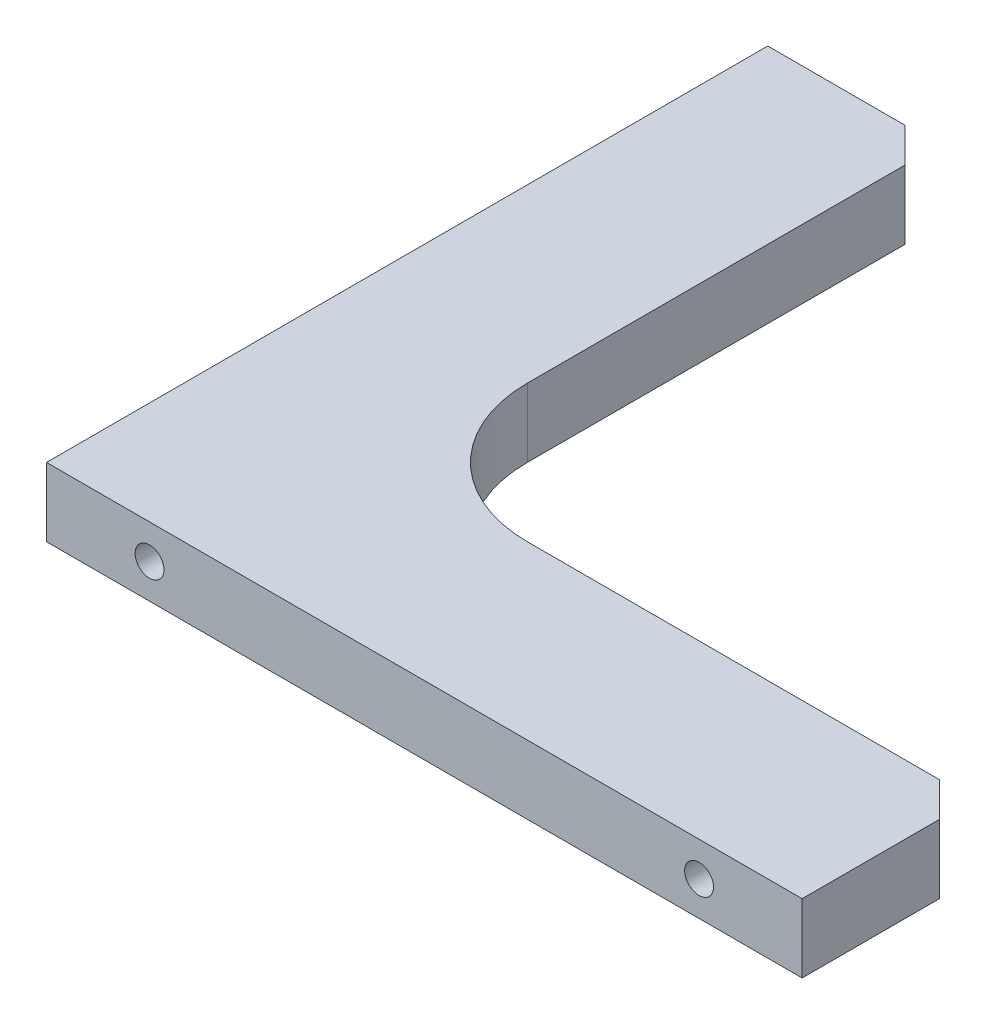
from build123d import *

# Parameters (mm, degrees)
SKETCH_1_W                  = 110
SKETCH_1_H                  = 105
EXTRUDE_1_DEPTH             = 5
CUT_EXTRUDE_1_DEPTH         = 10
CHAMFER_1_SIZE              = 5
HOLE_WIZARD_M5_1_AT_2_COUNT = 2
HOLE_WIZARD_M5_1_AT_2_PITCH = 80


with BuildPart() as part:
    # 草图1 → 凸台-拉伸1 (new, symmetric)
    with BuildSketch(Plane(origin=(0, 0, 0), x_dir=(1, 0, 0), z_dir=(0, 1, 0))):
        Rectangle(SKETCH_1_W, SKETCH_1_H)
    extrude(amount=EXTRUDE_1_DEPTH, both=True)

    # 草图2 → 切除-拉伸1 (cut)
    with BuildSketch(Plane(origin=(0, 5, 0), x_dir=(1, 0, 0), z_dir=(0, 1, 0))):
        with BuildLine():
            Line((55, 52.5), (-30, 52.5))
            Line((-30, 52.5), (-30, -7.5))
            ThreePointArc((-30, -7.5), (-24.142135624, -21.642135624), (-10, -27.5))
            Line((-10, -27.5), (55, -27.5))
            Line((55, -27.5), (55, 52.5))
        make_face()
    extrude(amount=-CUT_EXTRUDE_1_DEPTH, mode=Mode.SUBTRACT)

    # 倒角1
    chamfer_1_edges = [part.edges().sort_by_distance(p)[0] for p in [
        (-30, 0, -52.5),
        (55, 0, 27.5),
    ]]
    chamfer(chamfer_1_edges, length=CHAMFER_1_SIZE)

    # 草图4 → M5 螺纹孔1 (revolve, cut)
    with BuildSketch(Plane(origin=(-55, 0, 37.5), x_dir=(0, 0, 1), z_dir=(0, 1, 0))):
        Polygon((0, 0), (0, 13.6618073), (2.1, 12.4), (2.1, 0), align=None)
    hole_wizard_m5_1 = revolve(axis=Axis((-61.35, 0, 37.5), (1, 0, 0)), mode=Mode.SUBTRACT)

    # M5 螺纹孔1 at 2: M5 螺纹孔1 ×2
    with Locations(*[(0, 0, -i * HOLE_WIZARD_M5_1_AT_2_PITCH) for i in range(1, HOLE_WIZARD_M5_1_AT_2_COUNT)]):
        add(hole_wizard_m5_1, mode=Mode.SUBTRACT)

    # 镜向1: M5 螺纹孔1 across plane
    add(hole_wizard_m5_1.mirror(Plane(origin=(-1.25, 0, -1.25), x_dir=(-0.7071067811865478, 0, 0.7071067811865472), z_dir=(-0.7071067811865475, 0, -0.7071067811865477))), mode=Mode.SUBTRACT)

    # 镜向1 copy 1 sketch → 镜向1 copy 1 (revolve, cut)
    with BuildSketch(Plane(origin=(40, 0, 52.5), x_dir=(-1, 0, 0), z_dir=(0, 1, 0))):
        Polygon((0, 0), (0, -13.6618073), (2.1, -12.4), (2.1, 0), align=None)
    revolve(axis=Axis((40, 0, 58.85), (0, 0, 1)), mode=Mode.SUBTRACT)


solid = part.part
